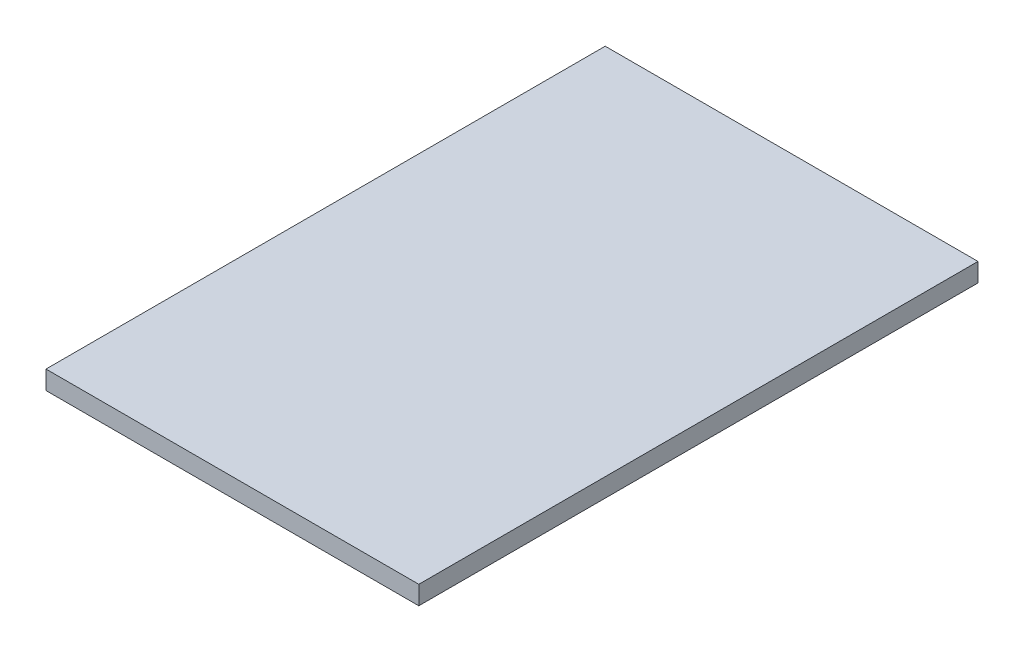
SolidWorks part; units mm, degrees
ref_plane "Front Plane" through (0, 0, 0) normal (0, 0, 1) x (1, 0, 0)
ref_plane "Top Plane" through (0, 0, 0) normal (0, 1, 0) x (1, 0, 0)
ref_plane "Right Plane" through (0, 0, 0) normal (1, 0, 0) x (0, 0, -1)
sketch "Sketch2" plane through (0, 0, 0) normal (0, 1, 0) x (1, 0, 0)
  line L1 (100, -150) -> (-100, -150)
  line L2 (100, -150) -> (100, 150)
  line L3 (100, 150) -> (-100, 150)
  line L4 (-100, -150) -> (-100, 150)
  line L5 (0, 150) -> (0, -150) construction
  line L6 (100, 0) -> (-100, 0) construction
  point P0 (0, 0)
  dimension "D1" = 200
  dimension "D2" = 300
extrude "Boss-Extrude1" add sketch "Sketch2" along normal blind 10
